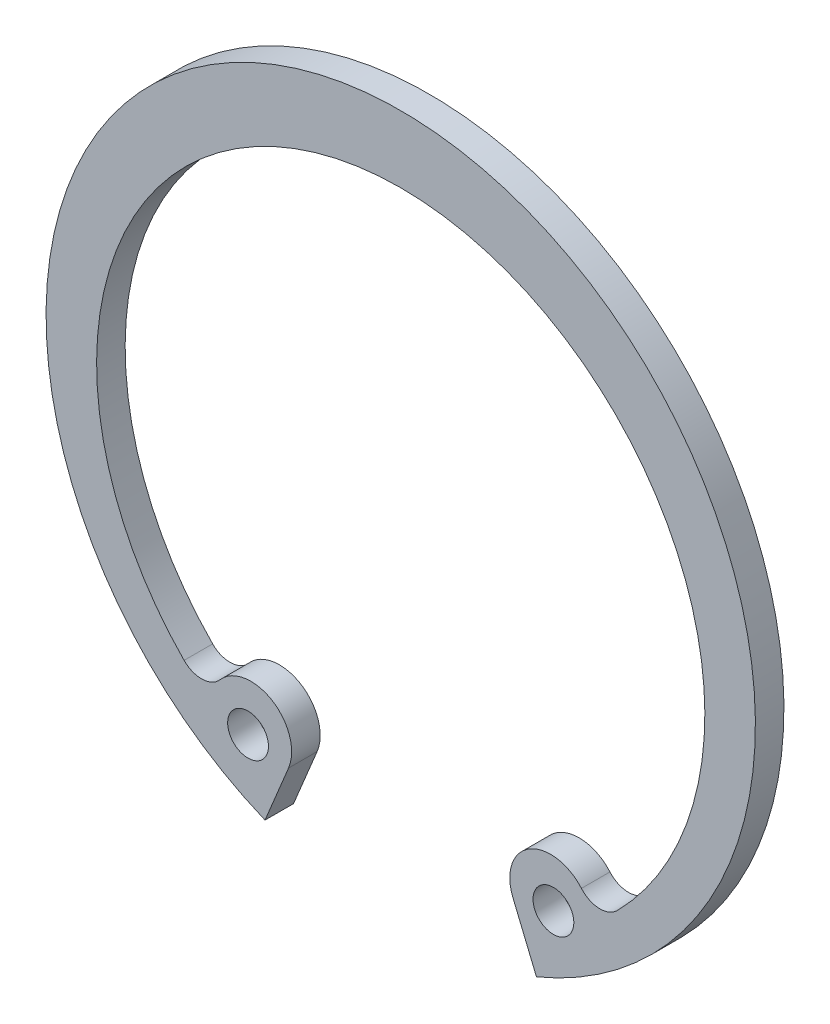
from build123d import *

# Parameters (mm, degrees)
SKETCH1_R          = 1.25
BASE_EXTRUDE_DEPTH = 1.75


with BuildPart() as part:
    # Sketch1 → Base-Extrude (new body)
    with BuildSketch(Plane.XY):
        with BuildLine():
            Line((-6.879499755, -16.608581611), (-8.323364654, -20.094379832))
            ThreePointArc((-8.323364654, -20.094379832), (0, 21.75), (8.323364654, -20.094379832))
            Line((8.323364654, -20.094379832), (6.879499755, -16.608581611))
            ThreePointArc((6.879499755, -16.608581611), (7.876948304, -13.523963446), (11.081029231, -14.017560694))
            ThreePointArc((11.081029231, -14.017560694), (12.16700015, -14.536168573), (13.28459359, -14.08976979))
            ThreePointArc((13.28459359, -14.08976979), (0, 17.65), (-13.28459359, -14.08976979))
            ThreePointArc((-13.28459359, -14.08976979), (-12.16700015, -14.536168573), (-11.081029231, -14.017560694))
            ThreePointArc((-11.081029231, -14.017560694), (-7.876948304, -13.523963446), (-6.879499755, -16.608581611))
        make_face()
        with Locations((-9.363022706, -16.071521577)):
            Circle(SKETCH1_R, mode=Mode.SUBTRACT)
        with Locations(Location((9.363022706, -16.071521577, 0), (0, 0, 180))):
            Circle(SKETCH1_R, mode=Mode.SUBTRACT)
    extrude(amount=BASE_EXTRUDE_DEPTH)


solid = part.part
